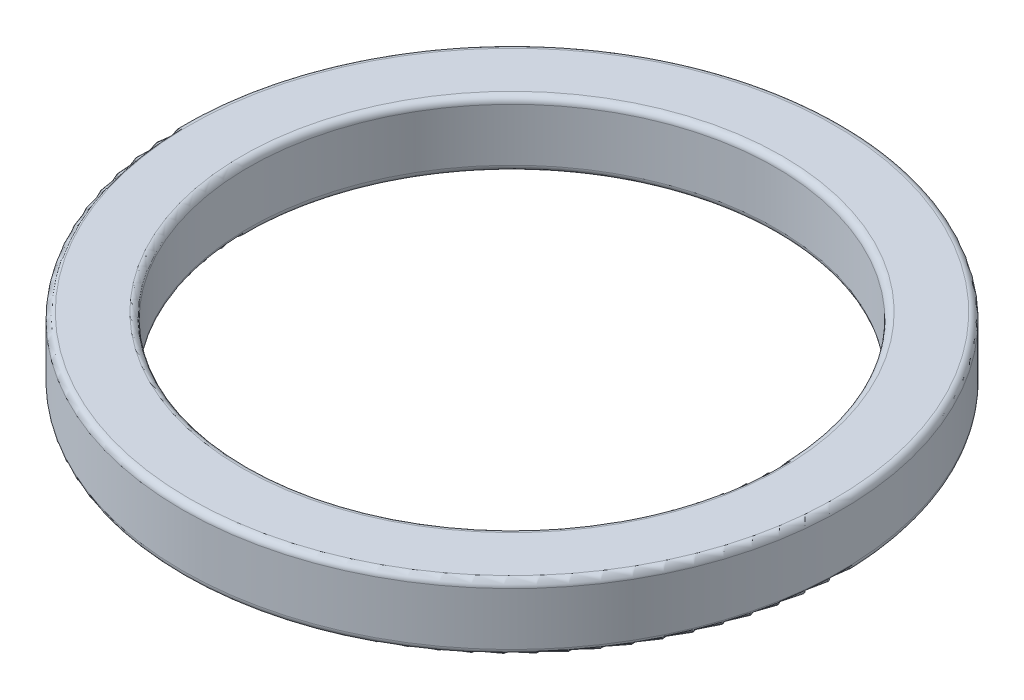
from build123d import *

# Parameters (mm, degrees)
SKETCH_1_R      = 50
SKETCH_1_R_2    = 40
EXTRUDE_1_DEPTH = 10
FILLET_1_R      = 1


with BuildPart() as part:
    # 草图1 → 凸台-拉伸1 (new body)
    with BuildSketch(Plane(origin=(0, 0, 0), x_dir=(1, 0, 0), z_dir=(0, 1, 0))):
        with Locations(Location((0, 0, 0), (0, 0, 270))):
            Circle(SKETCH_1_R)
        with Locations(Location((0, 0, 0), (0, 0, 270))):
            Circle(SKETCH_1_R_2, mode=Mode.SUBTRACT)
    extrude(amount=EXTRUDE_1_DEPTH)

    # 圆角1
    fillet_1_edges = [part.edges().sort_by_distance(p)[0] for p in [
        (0, 0, -50),
        (0, 10, -50),
        (0, 0, -40),
        (0, 10, -40),
    ]]
    fillet(fillet_1_edges, radius=FILLET_1_R)


solid = part.part
